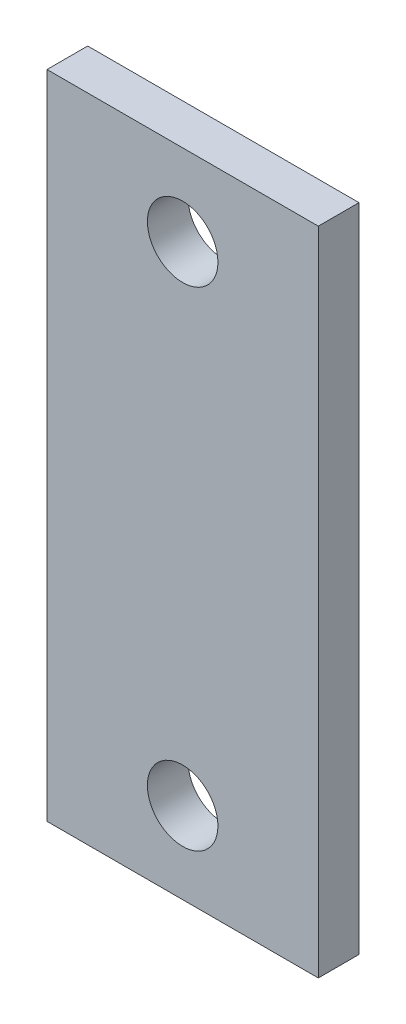
SolidWorks part; units mm, degrees
material "Q235-A"
ref_plane "Front Plane" through (0, 0, 0) normal (0, 0, 1) x (1, 0, 0)
ref_plane "Top Plane" through (0, 0, 0) normal (0, 1, 0) x (1, 0, 0)
ref_plane "Right Plane" through (0, 0, 0) normal (1, 0, 0) x (0, 0, -1)
sketch "Sketch1" plane through (0, 0, 0) normal (0, 0, 1) x (1, 0, 0)
  line L1 (50, -120) -> (-50, -120)
  line L2 (50, -120) -> (50, 120)
  line L3 (50, 120) -> (-50, 120)
  line L4 (-50, -120) -> (-50, 120)
  line L5 (50, -120) -> (-50, 120) construction
  line L6 (50, 120) -> (-50, -120) construction
  point P0 (0, 0)
  dimension "D1" = 240
  dimension "D2" = 100
extrude "Boss-Extrude1" add sketch "Sketch1" along normal mid plane 15
sketch "Sketch2" plane through (0, 0, 7.5) normal (0, 0, 1) x (1, 0, 0)
  line L0 (0, -90) -> (0, 90) construction
  circle A0 centre (0, 90) radius 13
  circle A1 centre (0, -90) radius 13
  point P4 (0, 0)
  dimension "D1" = 180
  dimension "D2" = 26
extrude "Cut-Extrude1" cut sketch "Sketch2" against normal blind 32
